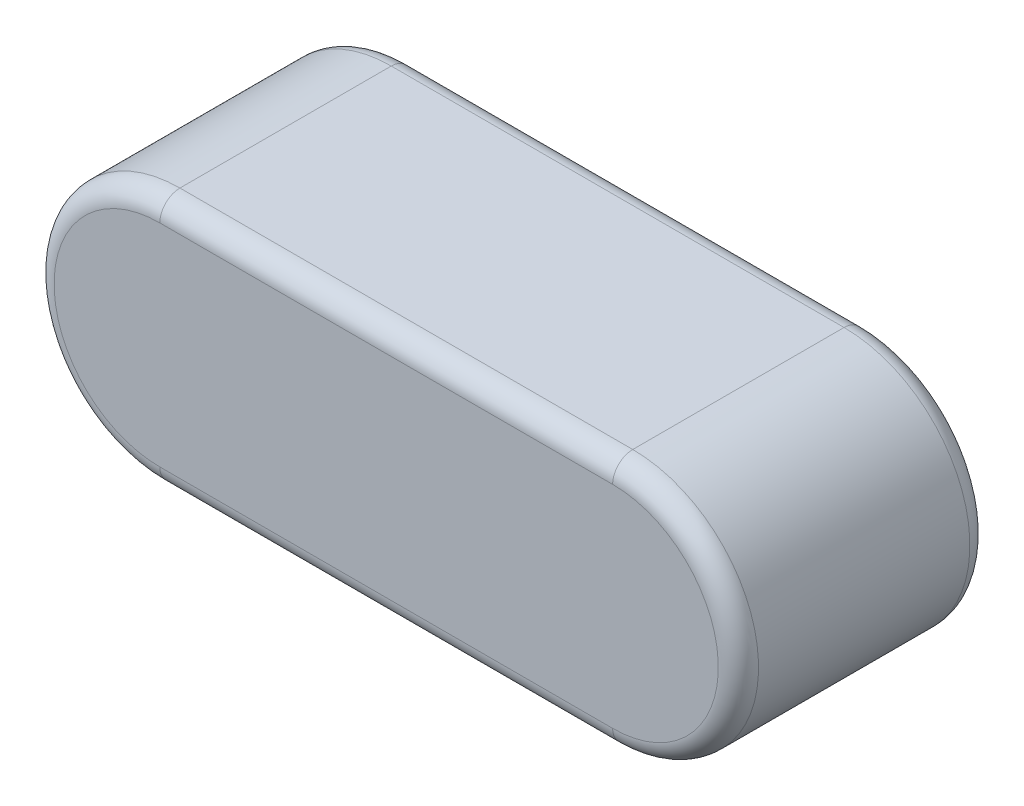
from build123d import *

# Parameters (mm, degrees)
EXTRUDE_527_DEPTH = 5
FILLET_1_R        = 0.4


with BuildPart() as part:
    # 草图1 → Extrude 527 (new body)
    with BuildSketch(Plane.XY):
        with BuildLine():
            Line((-4.5, 2.5), (4.5, 2.5))
            ThreePointArc((4.5, 2.5), (7, 0), (4.5, -2.5))
            Line((4.5, -2.5), (-4.5, -2.5))
            ThreePointArc((-4.5, -2.5), (-7, 0), (-4.5, 2.5))
        make_face()
    extrude(amount=EXTRUDE_527_DEPTH)

    # 圆角1
    fillet_1_edges = [part.edges().sort_by_distance(p)[0] for p in [
        (7, 0, 5),
        (0, 2.5, 5),
        (-7, 0, 5),
        (0, 2.5, 0),
        (7, 0, 0),
        (0, -2.5, 0),
        (-7, 0, 0),
        (0, -2.5, 5),
    ]]
    fillet(fillet_1_edges, radius=FILLET_1_R)


solid = part.part
